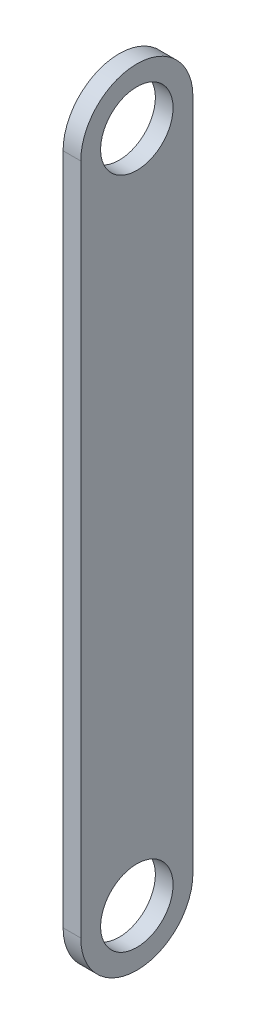
SolidWorks part; units mm, degrees
ref_plane "Front Plane" through (0, 0, 0) normal (0, 0, 1) x (1, 0, 0)
ref_plane "Top Plane" through (0, 0, 0) normal (0, 1, 0) x (1, 0, 0)
ref_plane "Right Plane" through (0, 0, 0) normal (1, 0, 0) x (0, 0, -1)
sketch "Sketch1" plane through (0, 0, 0) normal (1, 0, 0) x (0, 0, -1)
  line L0 (0, -38.1) -> (0, 38.1) construction
  line L1 (-6.35, -38.1) -> (-6.35, 38.1)
  line L2 (6.35, -38.1) -> (6.35, 38.1)
  arc A0 (-6.35, -38.1) -> (6.35, -38.1) centre (0, -38.1) ccw
  arc A1 (6.35, 38.1) -> (-6.35, 38.1) centre (0, 38.1) ccw
  circle A2 centre (0, 38.1) radius 4.1
  circle A3 centre (0, -38.1) radius 4.1
  point P2 (0, 0)
  dimension "D3" = 8.2
  dimension "D1" = 76.2
  dimension "D2" = 12.7
extrude "Boss-Extrude1" add sketch "Sketch1" along normal blind 2
